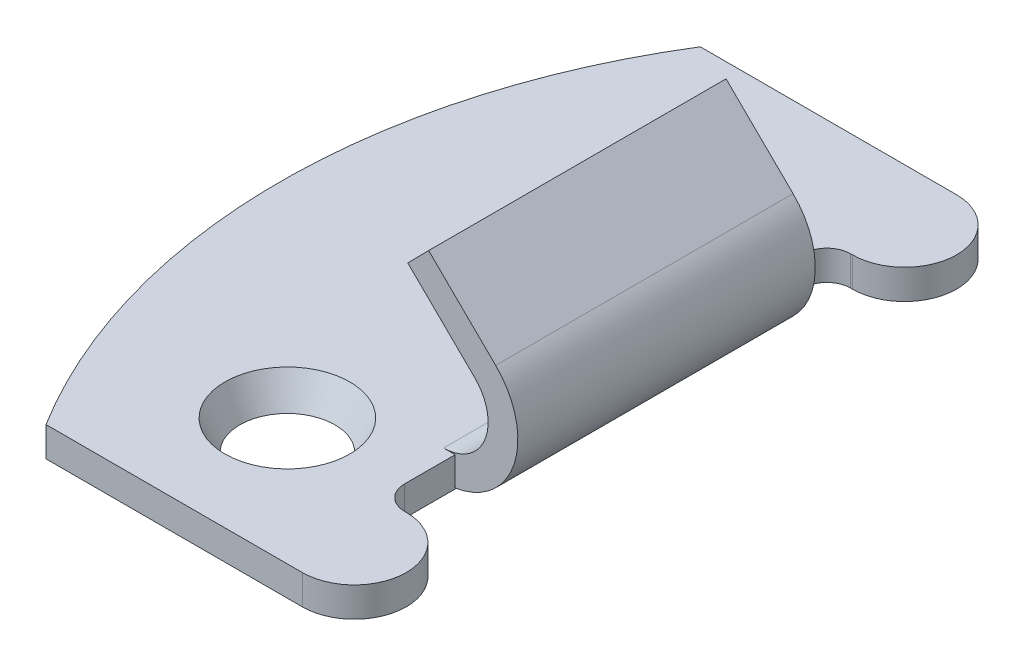
from build123d import *

# Parameters (mm, degrees)
BOSS_EXTRUDE1_DEPTH      = 5
BOSS_EXTRUDE1_DEPTH_BACK = 5
BOSS_EXTRUDE2_DEPTH      = 1
SKETCH3_W                = 100
SKETCH3_H                = 100
SKETCH3_R                = 20.87
CUT_EXTRUDE1_DEPTH       = 2


with BuildPart() as part:
    # Sketch1 → Boss-Extrude1 (new, two sides: drawn at the far end of the back side and taken through both)
    with BuildSketch(Plane.XY.offset(-BOSS_EXTRUDE1_DEPTH_BACK)):
        with BuildLine():
            Line((0, 0), (10.5, 0))
            ThreePointArc((10.5, 0), (12.813469706, 1.552446351), (12.253709329, 4.281713666))
            Line((12.253709329, 4.281713666), (10, 6.5))
            Line((10, 6.5), (9.298516268, 5.787314534))
            Line((9.298516268, 5.787314534), (11.552225598, 3.5690282))
            ThreePointArc((11.552225598, 3.5690282), (11.888081824, 1.931467811), (10.5, 1))
            Line((10.5, 1), (0, 1))
            Line((0, 1), (0, 0))
        make_face()
    extrude(amount=BOSS_EXTRUDE1_DEPTH + BOSS_EXTRUDE1_DEPTH_BACK)

    # Sketch2 → Boss-Extrude2 (add)
    with BuildSketch(Plane(origin=(0, 0, 0), x_dir=(1, 0, 0), z_dir=(0, 1, 0))):
        with BuildLine():
            Line((3.134247972, -11), (11.75, -11))
            ThreePointArc((11.75, -11), (13.5, -9.25), (11.75, -7.5))
            Line((11.75, -7.5), (11.69, -7.5))
            ThreePointArc((11.69, -7.5), (11.124314575, -7.265685425), (10.89, -6.7))
            Line((10.89, -6.7), (10.89, 6.7))
            ThreePointArc((10.89, 6.7), (11.124314575, 7.265685425), (11.69, 7.5))
            Line((11.69, 7.5), (11.75, 7.5))
            ThreePointArc((11.75, 7.5), (13.5, 9.25), (11.75, 11))
            Line((11.75, 11), (3.134247972, 11))
            ThreePointArc((3.134247972, 11), (0, 0), (3.134247972, -11))
        make_face()
    extrude(amount=BOSS_EXTRUDE2_DEPTH)

    # Sketch3 → Cut-Extrude1 (cut)
    with BuildSketch(Plane(origin=(0, 0, 0), x_dir=(1, 0, 0), z_dir=(0, 1, 0))):
        Rectangle(SKETCH3_W, SKETCH3_H)
        with Locations((20.87, 0)):
            Circle(SKETCH3_R, mode=Mode.SUBTRACT)
    extrude(amount=CUT_EXTRUDE1_DEPTH, mode=Mode.SUBTRACT)

    # Sketch4 → Cut-Revolve1 (revolve, cut)
    with BuildSketch(Plane.XY.offset(6.75), mode=Mode.PRIVATE) as cut_revolve1_sk:
        Polygon((7, 1), (9.1, 1), (8.6, 0), (7, 0), align=None)
    revolve(cut_revolve1_sk.sketch.rotate(Axis((7, 0, 6.75), (0, 1, 0)), 270), axis=Axis((7, 0, 6.75), (0, 1, 0)), mode=Mode.SUBTRACT)

    # Sketch5 → Cut-Revolve2 (revolve, cut)
    with BuildSketch(Plane.XY.offset(-6.75), mode=Mode.PRIVATE) as cut_revolve2_sk:
        Polygon((7, 1), (9.1, 1), (8.6, 0), (7, 0), align=None)
    revolve(cut_revolve2_sk.sketch.rotate(Axis((7, 0, -6.75), (0, 1, 0)), 270), axis=Axis((7, 0, -6.75), (0, 1, 0)), mode=Mode.SUBTRACT)


solid = part.part
